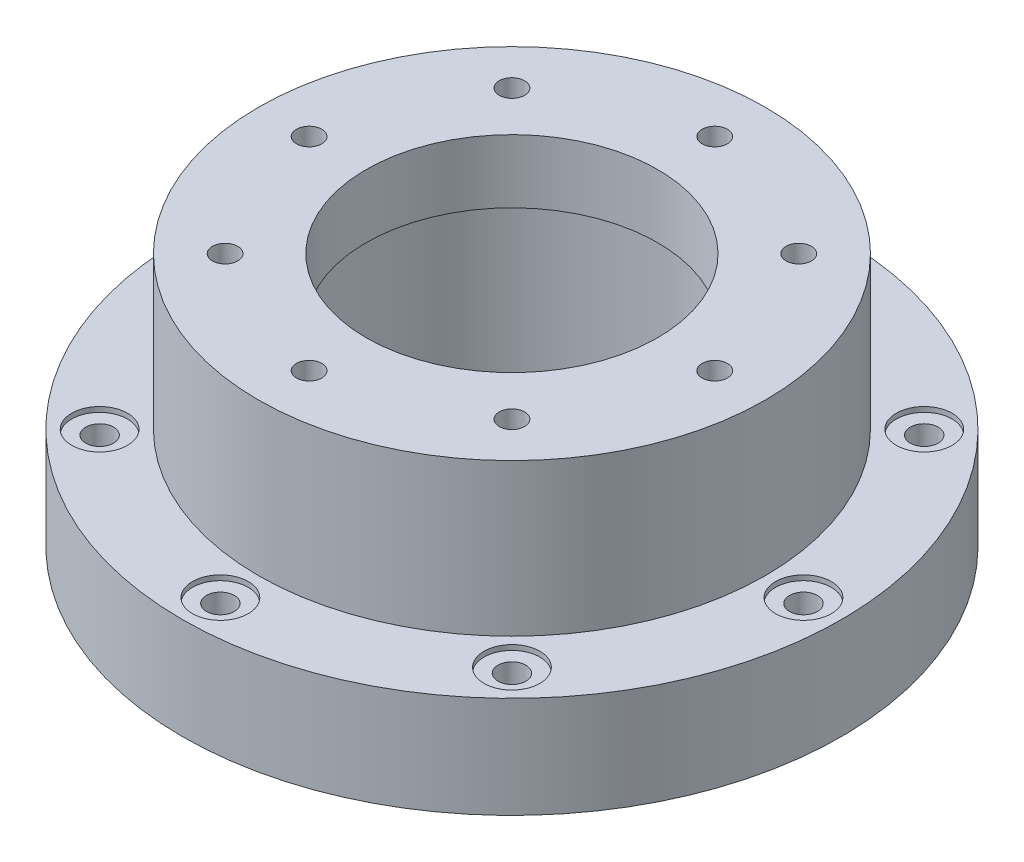
from build123d import *

# Parameters (mm, degrees)
SKETCH_2_R          = 11
CUT_EXTRUDE_1_DEPTH = 2
CUT_EXTRUDE_2_REACH = 196.342
SKETCH_3_R          = 5.5
SKETCH_4_R          = 5
CUT_EXTRUDE_3_DEPTH = 46


with BuildPart() as part:
    # 草图1 → 旋转1 (revolve)
    with BuildSketch(Plane.XY, mode=Mode.PRIVATE) as revolve_1_sk:
        with BuildLine():
            Line((65, 35), (57.5, 35))
            Line((57.5, 35), (57.5, 60))
            Line((57.5, 60), (100, 60))
            Line((100, 60), (100, 0))
            Line((100, 0), (130, 0))
            Line((130, 0), (130, -40))
            Line((130, -40), (87.5, -40))
            ThreePointArc((87.5, -40), (80.428932188, -42.928932188), (77.5, -50))
            Line((77.5, -50), (77.5, -65))
            Line((77.5, -65), (65, -65))
            Line((65, -65), (65, 35))
        make_face()
    revolve(revolve_1_sk.sketch.rotate(Axis((0, 133.6875, 0), (0, -1, 0)), 90), axis=Axis((0, 133.6875, 0), (0, -1, 0)))

    # 草图2 → 切除-拉伸1 (cut)
    with BuildSketch(Plane(origin=(0, 0, 0), x_dir=(1, 0, 0), z_dir=(0, 1, 0))):
        with Locations(Location((115, 0, 0), (0, 0, 270))):
            Circle(SKETCH_2_R)
        with Locations(Location((81.317279836, -81.317279836, 0), (0, 0, 270))):
            Circle(SKETCH_2_R)
        with Locations(Location((0, -115, 0), (0, 0, 270))):
            Circle(SKETCH_2_R)
        with Locations(Location((-81.317279836, -81.317279836, 0), (0, 0, 270))):
            Circle(SKETCH_2_R)
        with Locations(Location((-115, 0, 0), (0, 0, 270))):
            Circle(SKETCH_2_R)
        with Locations(Location((-81.317279836, 81.317279836, 0), (0, 0, 270))):
            Circle(SKETCH_2_R)
        with Locations(Location((0, 115, 0), (0, 0, 270))):
            Circle(SKETCH_2_R)
        with Locations(Location((81.317279836, 81.317279836, 0), (0, 0, 270))):
            Circle(SKETCH_2_R)
    extrude(amount=-CUT_EXTRUDE_1_DEPTH, mode=Mode.SUBTRACT)

    # 草图3 → 切除-拉伸2 (cut, up to next)
    with BuildSketch(Plane(origin=(0, -2, 0), x_dir=(1, 0, 0), z_dir=(0, 1, 0)), mode=Mode.PRIVATE) as cut_extrude_2_sk1:
        with Locations(Location((81.317279836, 81.317279836, 0), (0, 0, 270))):
            Circle(SKETCH_3_R)
    cut_extrude_2_tool1 = extrude(cut_extrude_2_sk1.sketch, amount=-CUT_EXTRUDE_2_REACH, mode=Mode.PRIVATE) & part.part
    # 草图3 → 切除-拉伸2 (cut, up to next)
    with BuildSketch(Plane(origin=(0, -2, 0), x_dir=(1, 0, 0), z_dir=(0, 1, 0)), mode=Mode.PRIVATE) as cut_extrude_2_sk2:
        with Locations(Location((115, 0, 0), (0, 0, 270))):
            Circle(SKETCH_3_R)
    cut_extrude_2_tool2 = extrude(cut_extrude_2_sk2.sketch, amount=-CUT_EXTRUDE_2_REACH, mode=Mode.PRIVATE) & part.part
    # 草图3 → 切除-拉伸2 (cut, up to next)
    with BuildSketch(Plane(origin=(0, -2, 0), x_dir=(1, 0, 0), z_dir=(0, 1, 0)), mode=Mode.PRIVATE) as cut_extrude_2_sk3:
        with Locations(Location((81.317279836, -81.317279836, 0), (0, 0, 270))):
            Circle(SKETCH_3_R)
    cut_extrude_2_tool3 = extrude(cut_extrude_2_sk3.sketch, amount=-CUT_EXTRUDE_2_REACH, mode=Mode.PRIVATE) & part.part
    # 草图3 → 切除-拉伸2 (cut, up to next)
    with BuildSketch(Plane(origin=(0, -2, 0), x_dir=(1, 0, 0), z_dir=(0, 1, 0)), mode=Mode.PRIVATE) as cut_extrude_2_sk4:
        with Locations(Location((0, -115, 0), (0, 0, 270))):
            Circle(SKETCH_3_R)
    cut_extrude_2_tool4 = extrude(cut_extrude_2_sk4.sketch, amount=-CUT_EXTRUDE_2_REACH, mode=Mode.PRIVATE) & part.part
    # 草图3 → 切除-拉伸2 (cut, up to next)
    with BuildSketch(Plane(origin=(0, -2, 0), x_dir=(1, 0, 0), z_dir=(0, 1, 0)), mode=Mode.PRIVATE) as cut_extrude_2_sk5:
        with Locations(Location((-81.317279836, -81.317279836, 0), (0, 0, 270))):
            Circle(SKETCH_3_R)
    cut_extrude_2_tool5 = extrude(cut_extrude_2_sk5.sketch, amount=-CUT_EXTRUDE_2_REACH, mode=Mode.PRIVATE) & part.part
    # 草图3 → 切除-拉伸2 (cut, up to next)
    with BuildSketch(Plane(origin=(0, -2, 0), x_dir=(1, 0, 0), z_dir=(0, 1, 0)), mode=Mode.PRIVATE) as cut_extrude_2_sk6:
        with Locations(Location((-115, 0, 0), (0, 0, 270))):
            Circle(SKETCH_3_R)
    cut_extrude_2_tool6 = extrude(cut_extrude_2_sk6.sketch, amount=-CUT_EXTRUDE_2_REACH, mode=Mode.PRIVATE) & part.part
    # 草图3 → 切除-拉伸2 (cut, up to next)
    with BuildSketch(Plane(origin=(0, -2, 0), x_dir=(1, 0, 0), z_dir=(0, 1, 0)), mode=Mode.PRIVATE) as cut_extrude_2_sk7:
        with Locations(Location((-81.317279836, 81.317279836, 0), (0, 0, 270))):
            Circle(SKETCH_3_R)
    cut_extrude_2_tool7 = extrude(cut_extrude_2_sk7.sketch, amount=-CUT_EXTRUDE_2_REACH, mode=Mode.PRIVATE) & part.part
    # 草图3 → 切除-拉伸2 (cut, up to next)
    with BuildSketch(Plane(origin=(0, -2, 0), x_dir=(1, 0, 0), z_dir=(0, 1, 0)), mode=Mode.PRIVATE) as cut_extrude_2_sk8:
        with Locations(Location((0, 115, 0), (0, 0, 270))):
            Circle(SKETCH_3_R)
    cut_extrude_2_tool8 = extrude(cut_extrude_2_sk8.sketch, amount=-CUT_EXTRUDE_2_REACH, mode=Mode.PRIVATE) & part.part
    add(cut_extrude_2_tool1.solids().sort_by_distance((81.31728, -2, -81.31728))[0], mode=Mode.SUBTRACT)
    add(cut_extrude_2_tool2.solids().sort_by_distance((115, -2, 0))[0], mode=Mode.SUBTRACT)
    add(cut_extrude_2_tool3.solids().sort_by_distance((81.31728, -2, 81.31728))[0], mode=Mode.SUBTRACT)
    add(cut_extrude_2_tool4.solids().sort_by_distance((0, -2, 115))[0], mode=Mode.SUBTRACT)
    add(cut_extrude_2_tool5.solids().sort_by_distance((-81.31728, -2, 81.31728))[0], mode=Mode.SUBTRACT)
    add(cut_extrude_2_tool6.solids().sort_by_distance((-115, -2, 0))[0], mode=Mode.SUBTRACT)
    add(cut_extrude_2_tool7.solids().sort_by_distance((-81.31728, -2, -81.31728))[0], mode=Mode.SUBTRACT)
    add(cut_extrude_2_tool8.solids().sort_by_distance((0, -2, -115))[0], mode=Mode.SUBTRACT)

    # 草图4 → 切除-拉伸3 (cut)
    with BuildSketch(Plane(origin=(0, 60, 0), x_dir=(1, 0, 0), z_dir=(0, 1, 0))):
        with Locations(Location((80, 0, 0), (0, 0, 270))):
            Circle(SKETCH_4_R)
        with Locations(Location((56.568542495, -56.568542495, 0), (0, 0, 270))):
            Circle(SKETCH_4_R)
        with Locations(Location((0, -80, 0), (0, 0, 270))):
            Circle(SKETCH_4_R)
        with Locations(Location((-56.568542495, -56.568542495, 0), (0, 0, 270))):
            Circle(SKETCH_4_R)
        with Locations(Location((-80, 0, 0), (0, 0, 270))):
            Circle(SKETCH_4_R)
        with Locations(Location((-56.568542495, 56.568542495, 0), (0, 0, 270))):
            Circle(SKETCH_4_R)
        with Locations(Location((0, 80, 0), (0, 0, 270))):
            Circle(SKETCH_4_R)
        with Locations(Location((56.568542495, 56.568542495, 0), (0, 0, 270))):
            Circle(SKETCH_4_R)
    extrude(amount=-CUT_EXTRUDE_3_DEPTH, mode=Mode.SUBTRACT)


solid = part.part
